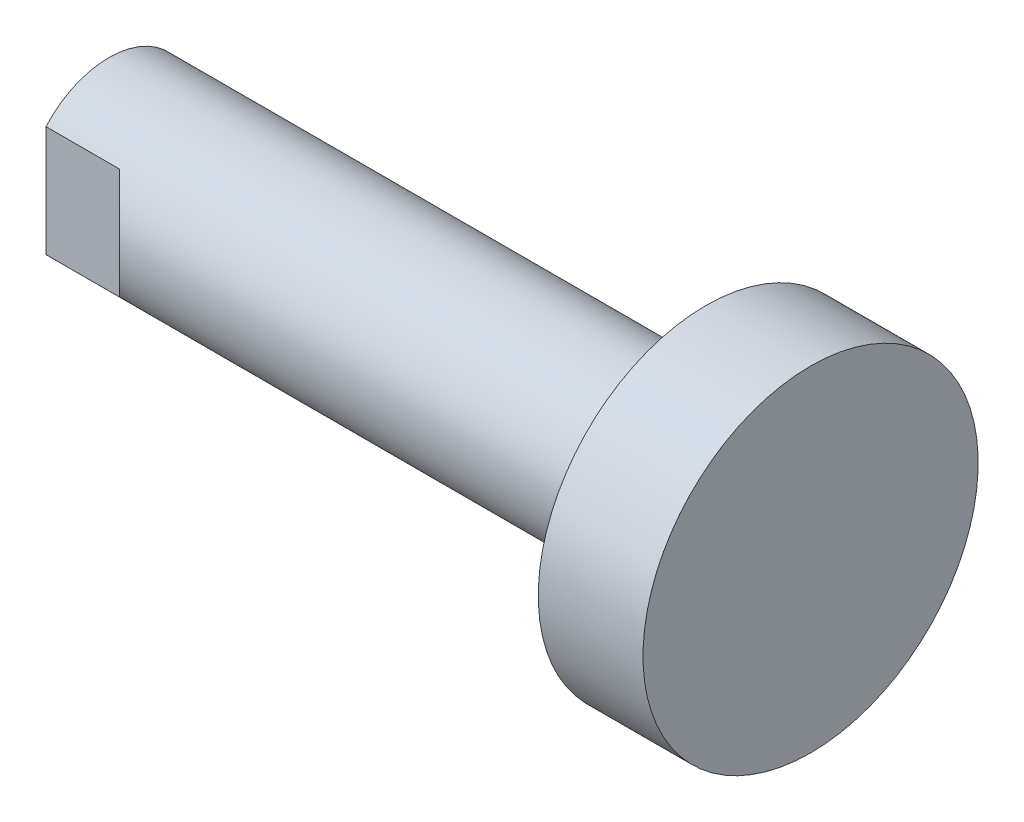
from build123d import *

# Parameters (mm, degrees)
CUT_EXTRUDE1_DEPTH      = 8
CUT_EXTRUDE1_DEPTH_BACK = 8


with BuildPart() as part:
    # Sketch1 → Revolve1 (revolve)
    with BuildSketch(Plane.XY, mode=Mode.PRIVATE) as revolve1_sk:
        Polygon((5.435884786, 0), (4.5, 1.621), (-3.121, 1.621), (-3.5, 2), (-3.5, 4), (25, 4), (25, 8), (30, 8), (30, 0), align=None)
    revolve(revolve1_sk.sketch.rotate(Axis((30, 0, 0), (-1, 0, 0)), 180), axis=Axis((30, 0, 0), (-1, 0, 0)))

    # Sketch2 → Cut-Extrude1 (cut, two sides: drawn at the far end of the back side and taken through both)
    with BuildSketch(Plane(origin=(0, 0, 0), x_dir=(1, 0, 0), z_dir=(0, 1, 0)).offset(-CUT_EXTRUDE1_DEPTH_BACK)):
        Polygon((-8.5, 8), (-8.5, -8), (5, -8), (0, -3), (-3.5, -3), (-3.5, 3), (0, 3), (5, 8), align=None)
    extrude(amount=CUT_EXTRUDE1_DEPTH + CUT_EXTRUDE1_DEPTH_BACK, mode=Mode.SUBTRACT)


solid = part.part
